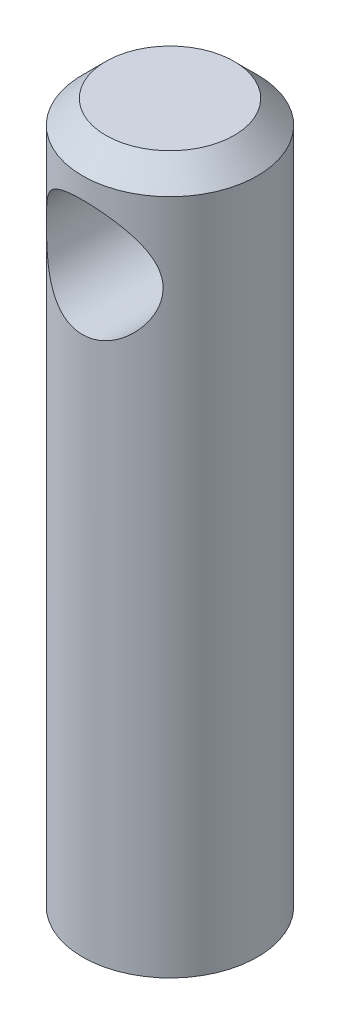
from build123d import *

# Parameters (mm, degrees)
SKETCH1_R               = 150
BOSS_EXTRUDE1_DEPTH     = 2400
CUT_EXTRUDE1_DEPTH      = 4000
CUT_EXTRUDE1_DEPTH_BACK = 4000
SKETCH2_R               = 100
SKETCH3_R               = 364.072238149
CUT_EXTRUDE2_DEPTH      = 1200
CHAMFER1_SIZE           = 40


with BuildPart() as part:
    # Sketch1 → Boss-Extrude1 (new body)
    with BuildSketch(Plane(origin=(0, 0, 0), x_dir=(1, 0, 0), z_dir=(0, 1, 0))):
        with Locations(Location((0, 0, 0), (0, 0, 270))):
            Circle(SKETCH1_R)
    extrude(amount=BOSS_EXTRUDE1_DEPTH)

    # Sketch2 → Cut-Extrude1 (cut, two sides: drawn at the far end of the back side and taken through both)
    with BuildSketch(Plane.XY.offset(-CUT_EXTRUDE1_DEPTH_BACK)):
        with Locations(Location((0, 2224.223653396, 0), (0, 0, 89.999999999))):
            Circle(SKETCH2_R)
    extrude(amount=CUT_EXTRUDE1_DEPTH + CUT_EXTRUDE1_DEPTH_BACK, mode=Mode.SUBTRACT)

    # Sketch3 → Cut-Extrude2 (cut)
    with BuildSketch(Plane.XZ):
        Circle(SKETCH3_R)
    extrude(amount=-CUT_EXTRUDE2_DEPTH, mode=Mode.SUBTRACT)

    # Chamfer1
    chamfer1_edges = [part.edges().sort_by_distance(p)[0] for p in [
        (0, 2400, -150),
    ]]
    chamfer(chamfer1_edges, length=CHAMFER1_SIZE)


solid = part.part
